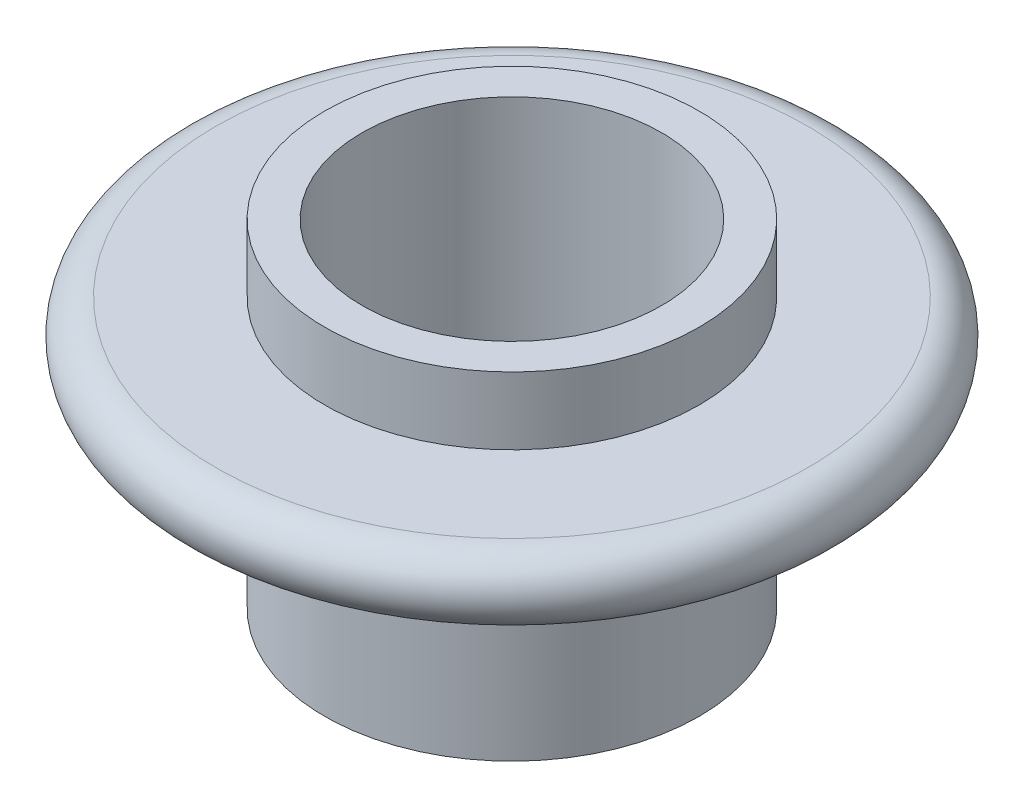
from build123d import *


with BuildPart() as part:
    # Sketch1 → Revolve1 (revolve)
    with BuildSketch(Plane.XY, mode=Mode.PRIVATE) as revolve1_sk:
        with BuildLine():
            Line((20, 22.5), (20, -22.5))
            Line((20, -22.5), (25, -22.5))
            Line((25, -22.5), (25, 4.5))
            Line((25, 4.5), (39.5, 4.5))
            ThreePointArc((39.5, 4.5), (44, 9), (39.5, 13.5))
            Line((39.5, 13.5), (25, 13.5))
            Line((25, 13.5), (25, 22.5))
            Line((25, 22.5), (20, 22.5))
        make_face()
    revolve(revolve1_sk.sketch.rotate(Axis((0, 22.5, 0), (0, -1, 0)), 180), axis=Axis((0, 22.5, 0), (0, -1, 0)))


solid = part.part
